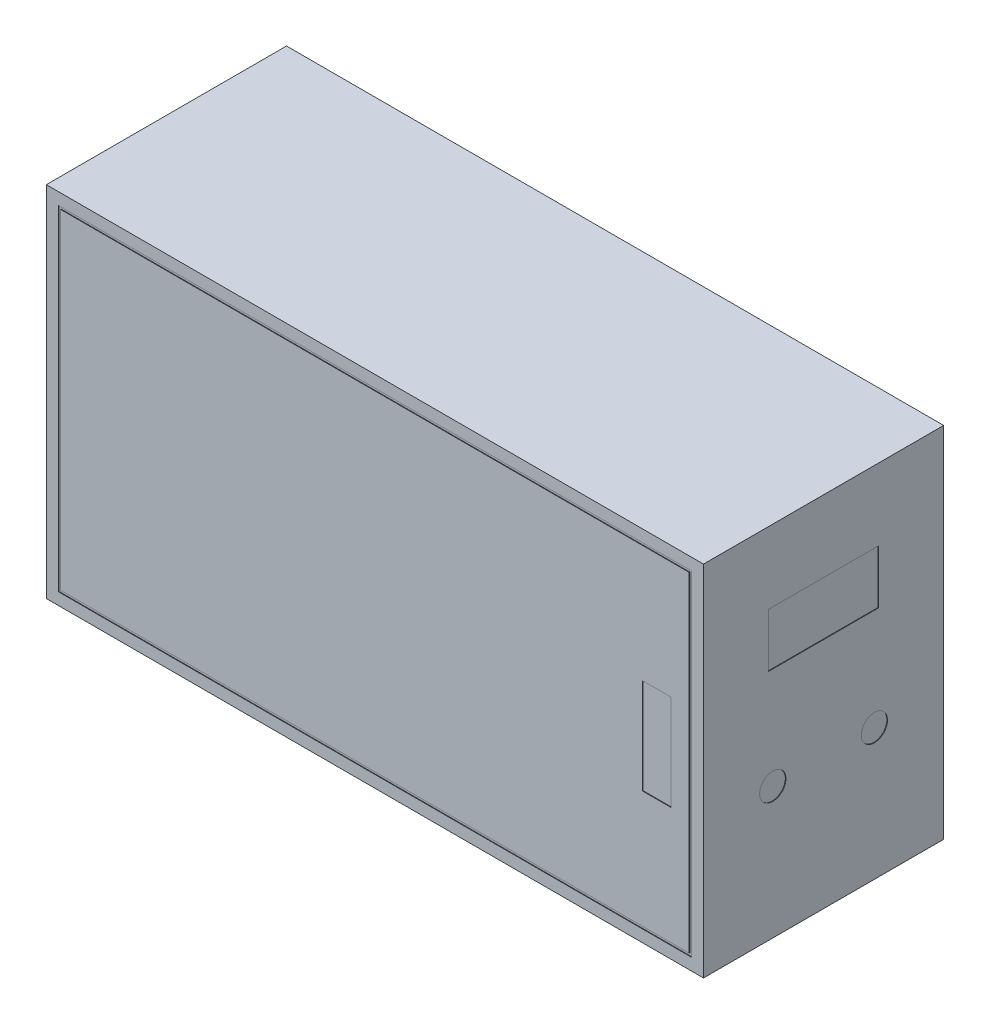
from build123d import *

# Parameters (mm, degrees)
SKETCH1_W           = 550
SKETCH1_H           = 300
BOSS_EXTRUDE1_DEPTH = 200
SHELL1_T            = -1.5
SKETCH2_W           = 550
SKETCH2_H           = 300
BOSS_EXTRUDE2_DEPTH = 1
SKETCH3_W           = 530
SKETCH3_H           = 280
SKETCH3_W_2         = 526
SKETCH3_H_2         = 276
SKETCH3_W_3         = 24
SKETCH3_H_3         = 80
CUT_EXTRUDE1_DEPTH  = 0.5
SKETCH5_R           = 11
SKETCH5_W           = 92
SKETCH5_H           = 45
CUT_EXTRUDE2_DEPTH  = 0.5


with BuildPart() as part:
    # Sketch1 → Boss-Extrude1 (new body)
    with BuildSketch(Plane.XY):
        with Locations((275, 150)):
            Rectangle(SKETCH1_W, SKETCH1_H)
    extrude(amount=BOSS_EXTRUDE1_DEPTH)

    # Shell1
    shell1_openings = [part.faces().sort_by_distance(p)[0] for p in [
        (275, 150, 200),
    ]]
    offset(amount=SHELL1_T, openings=shell1_openings, kind=Kind.INTERSECTION)

    # Sketch2 → Boss-Extrude2 (add)
    with BuildSketch(Plane.XY.offset(200)):
        with Locations((275, 150)):
            Rectangle(SKETCH2_W, SKETCH2_H)
    extrude(amount=BOSS_EXTRUDE2_DEPTH)

    # Sketch3 → Cut-Extrude1 (cut)
    # profile 1 of 2: a face of its own
    with BuildSketch(Plane.XY.offset(201)):
        with Locations((275, 150)):
            Rectangle(SKETCH3_W, SKETCH3_H)
        with Locations((275, 150)):
            Rectangle(SKETCH3_W_2, SKETCH3_H_2, mode=Mode.SUBTRACT)
    # profile 2 of 2: a face of its own
    with BuildSketch(Plane.XY.offset(201)):
        with Locations((511, 150)):
            Rectangle(SKETCH3_W_3, SKETCH3_H_3)
    extrude(amount=-CUT_EXTRUDE1_DEPTH, mode=Mode.SUBTRACT)

    # Sketch5 → Cut-Extrude2 (cut)
    with BuildSketch(Plane(origin=(550, 0, 0), x_dir=(0, 0, -1), z_dir=(1, 0, 0))):
        with Locations((-143, 110)):
            Circle(SKETCH5_R)
        with Locations((-58, 110)):
            Circle(SKETCH5_R)
        with Locations((-100.5, 217.5)):
            Rectangle(SKETCH5_W, SKETCH5_H)
    extrude(amount=-CUT_EXTRUDE2_DEPTH, mode=Mode.SUBTRACT)


solid = part.part
